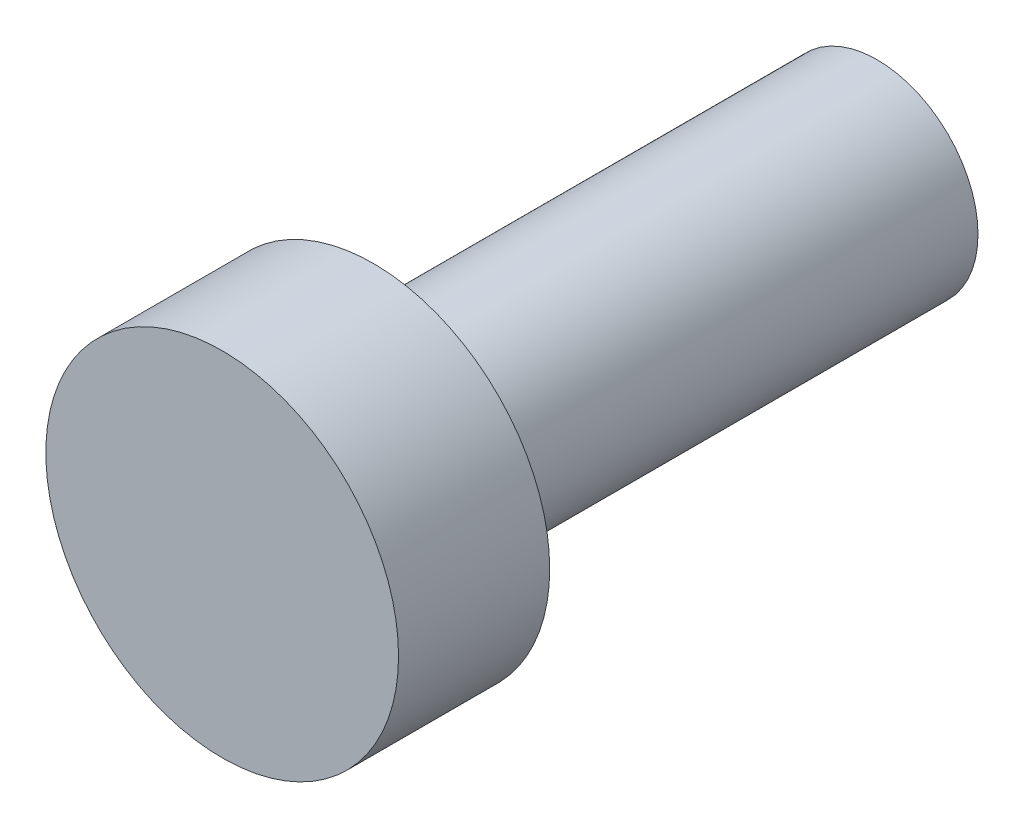
SolidWorks part; units mm, degrees
ref_plane "前视基准面" through (0, 0, 0) normal (0, 0, 1) x (1, 0, 0)
ref_plane "上视基准面" through (0, 0, 0) normal (0, 1, 0) x (1, 0, 0)
ref_plane "右视基准面" through (0, 0, 0) normal (1, 0, 0) x (0, 0, -1)
other "Configuration Table"
sketch "草图1" plane through (0, 0, 0) normal (0, 0, 1) x (1, 0, 0)
  circle A0 centre (0, 0) radius 2
  point P0 (0, 0)
  dimension "D1" = 4
extrude "凸台-拉伸1" add sketch "草图1" against normal blind 10
sketch "草图2" plane through (0, 0, 0) normal (0, 0, 1) x (1, 0, 0)
  circle A0 centre (0, 0) radius 3.5
  point P0 (0, 0)
  dimension "D1" = 7
extrude "凸台-拉伸2" add sketch "草图2" along normal blind 3
